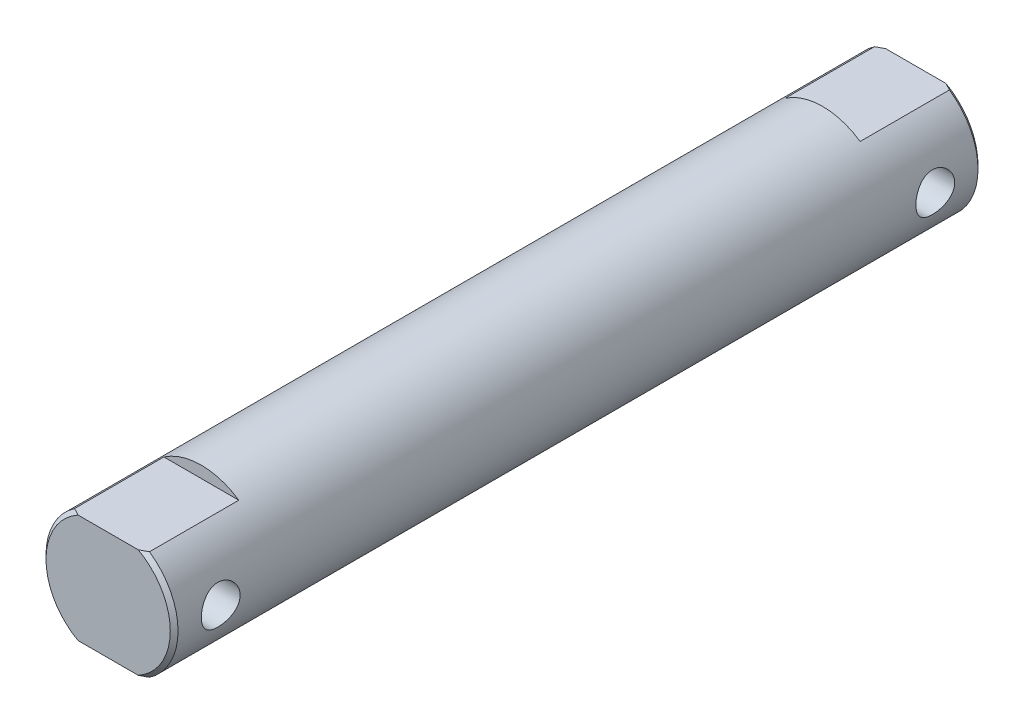
SolidWorks part; units mm, degrees
ref_plane "前视" through (0, 0, 0) normal (0, 0, 1) x (1, 0, 0)
ref_plane "上视" through (0, 0, 0) normal (0, 1, 0) x (1, 0, 0)
ref_plane "右视" through (0, 0, 0) normal (1, 0, 0) x (0, 0, -1)
sketch "草图1" plane through (0, 0, 0) normal (0, 0, 1) x (1, 0, 0)
  circle A0 centre (0, 0) radius 8.5
  dimension "D1" = 17
extrude "凸台-拉伸1" add sketch "草图1" along normal mid plane 104
sketch "草图2" plane through (0, 0, 52) normal (0, 0, 1) x (1, 0, 0)
  line L0 (0, 8.5) -> (0, -8.5) construction
  line L1 (-12.5, 10) -> (12.5, 10)
  line L2 (-12.5, 10) -> (-12.5, 7)
  line L3 (-12.5, 7) -> (12.5, 7)
  line L4 (12.5, 10) -> (12.5, 7)
  line L5 (-12.5, 10) -> (12.5, 7) construction
  line L6 (-12.5, 7) -> (12.5, 10) construction
  line L7 (0, 0) -> (8.5, 0) construction
  line L8 (-12.5, -7) -> (12.5, -10) construction
  line L9 (-12.5, -10) -> (12.5, -7) construction
  line L10 (12.5, -10) -> (12.5, -7)
  line L11 (-12.5, -7) -> (12.5, -7)
  line L12 (-12.5, -10) -> (-12.5, -7)
  line L13 (-12.5, -10) -> (12.5, -10)
  circle A0 centre (0, 0) radius 8.5 construction
  point P0 (0, 8.5)
  dimension "D1" = 25
  dimension "D2" = 14
extrude "切除-拉伸1" cut sketch "草图2" against normal blind 12
mirror "镜向1" about plane through (0, 0, 0) normal (0, 0, 1) of "切除-拉伸1"
chamfer "倒角2" distance 0.5 angle 45 4 edges at (8.5, 0, -52) (-8.5, 0, -52) (8.5, 0, 52) (-8.5, 0, 52)
ref_plane "基准面1" through (8.5, 0, 0) normal (1, 0, 0) x (0, 0, -1)
hole_wizard "M6 螺纹孔1" positions "草图4" profile "草图3" tap size "M6" standard "GB" end condition through all
sketch "草图4" plane through (8.5, 0, 0) normal (1, 0, 0) x (0, 0, -1)
  line L0 (-46, 0) -> (-52, 0) construction
  line L1 (-52, 7) -> (-52, -7) construction
  line L4 (46, 0) -> (52, 0) construction
  line L5 (52, -7) -> (52, 7) construction
  point P0 (-46, 0)
  point P2 (46, 0)
  dimension "D1" = 6
sketch "草图3" plane through (8.5, 0, 46) normal (0, 1, 0) x (0, 0, -1)
  line L0 (0, 0) -> (0, 17)
  line L1 (0, 17) -> (2.5, 17)
  line L2 (2.5, 17) -> (2.5, 0)
  line L5 (2.5, 0) -> (0, 0)
  line L11 (0, -6.35) -> (0, 107.95) construction
  dimension "通孔螺纹孔钻头直径" = 5
  dimension "通孔螺纹孔钻头深度" = 17
cosmetic thread "孔螺蚊线1" parameters "D2"=6
cosmetic thread "孔螺蚊线2" parameters "D2"=6
